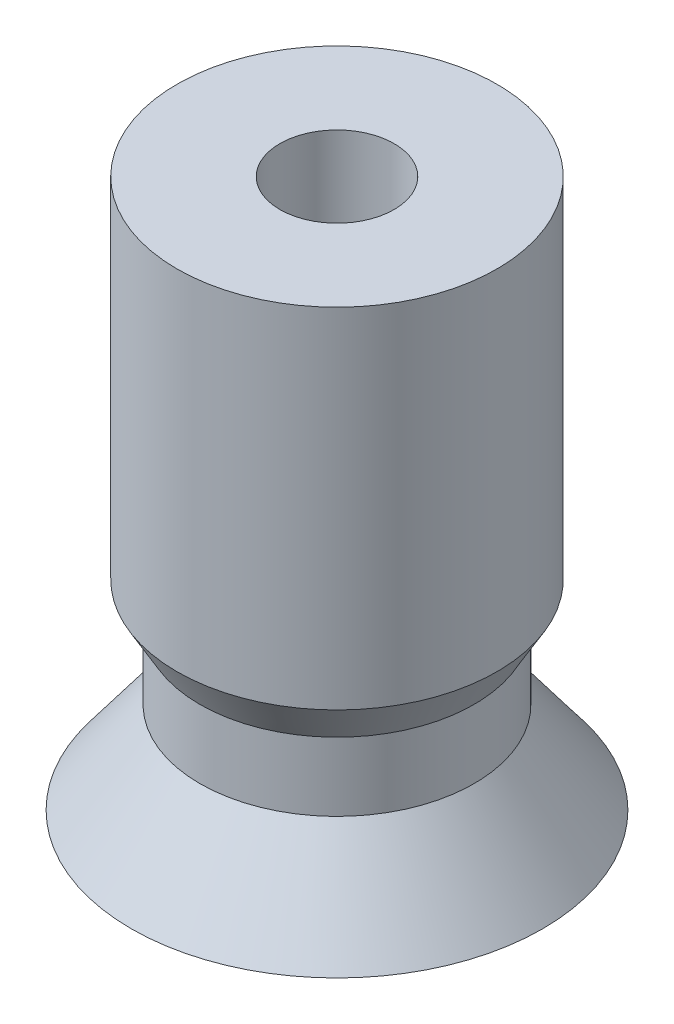
from build123d import *


with BuildPart() as part:
    # 草图1 → 旋转1 (revolve)
    with BuildSketch(Plane.XY, mode=Mode.PRIVATE) as revolve_1_sk:
        Polygon((1.25, 0), (4.5, 0), (3, 2), (3, 3.5), (3.5, 4.37), (3.5, 12), (1.25, 12), align=None)
    revolve(revolve_1_sk.sketch.rotate(Axis((0, 0, 0), (0, 1, 0)), 270), axis=Axis((0, 0, 0), (0, 1, 0)))


solid = part.part
